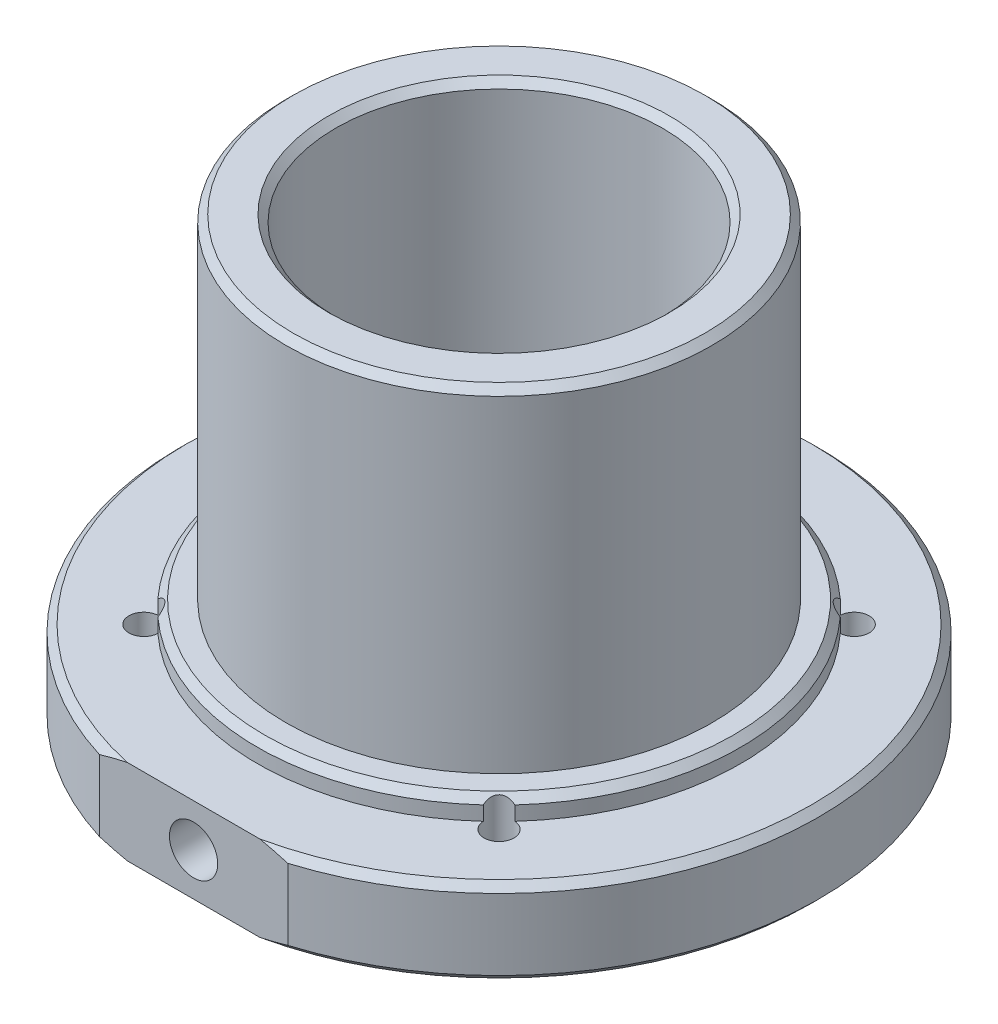
SolidWorks part; units mm, degrees
ref_plane "前视" through (0, 0, 0) normal (0, 0, 1) x (1, 0, 0)
ref_plane "上视" through (0, 0, 0) normal (0, 1, 0) x (1, 0, 0)
ref_plane "右视" through (0, 0, 0) normal (1, 0, 0) x (0, 0, -1)
sketch "草图1" plane through (0, 0, 0) normal (0, 1, 0) x (1, 0, 0)
  circle A0 centre (0, 0) radius 45
  dimension "D1" = 90
extrude "凸台-拉伸1" add sketch "草图1" along normal blind 12
sketch "草图2" plane through (0, 12, 0) normal (0, 1, 0) x (1, 0, 0)
  circle A0 centre (0, 0) radius 30
  dimension "D1" = 60
extrude "凸台-拉伸2" add sketch "草图2" along normal blind 50
cosmetic thread "装饰螺纹线1" parameters "D1"=20, "D2"=58.5
sketch "草图11" plane through (0, 12, 0) normal (0, 1, 0) x (1, 0, 0)
  circle A0 centre (0, 0) radius 34
  dimension "D1" = 68
extrude "凸台-拉伸3" add sketch "草图11" along normal blind 3
sketch "草图3" plane through (0, 0, 0) normal (0, -1, 0) x (1, 0, 0)
  circle A0 centre (0, 0) radius 23
  dimension "D1" = 46
extrude "切除-拉伸1" cut sketch "草图3" against normal through all
chamfer "倒角1" distance 1 angle 45 6 edges at (0, 0, 45) (0, 12, 45) (0, 62, 30) (0, 62, -23) (0, 0, -23) (0, 15, 34)
hole_wizard "M5 螺纹孔1" positions "草图5" profile "草图4" tap size "M5" standard "Gb" end condition through all
sketch "草图5" plane through (0, 0, 0) normal (0, -1, 0) x (-1, 0, 0)
  line L0 (0, 0) -> (0, -37.1797) construction
  line L2 (0, 0) -> (-51.8806, 0) construction
  point P0 (25, -25)
  point P2 (-25, -25)
  point P4 (-25, 25)
  point P6 (25, 25)
  dimension "D1" = 50
  dimension "D2" = 50
sketch "草图4" plane through (-25, 0, 25) normal (1, 0, 0) x (0, 0, -1)
  line L0 (0, 0) -> (0, 62)
  line L1 (0, 62) -> (2.1, 62)
  line L2 (2.1, 62) -> (2.1, 0)
  line L5 (2.1, 0) -> (0, 0)
  line L11 (0, -6.35) -> (0, 107.95) construction
  dimension "通孔螺纹孔钻头直径" = 4.2
  dimension "通孔螺纹孔钻头深度" = 62
cosmetic thread "孔螺蚊线1" parameters "D2"=5
cosmetic thread "孔螺蚊线2" parameters "D2"=5
cosmetic thread "孔螺蚊线3" parameters "D2"=5
cosmetic thread "孔螺蚊线4" parameters "D2"=5
sketch "草图8" plane through (0, 0, 0) normal (0, -1, 0) x (1, 0, 0)
  line L0 (-13.2665, 43) -> (13.2665, 43)
  circle A1 centre (0, 0) radius 45 construction
  arc A2 (13.2665, 43) -> (-13.2665, 43) centre (0, 0) ccw
  dimension "D1" = 43
extrude "切除-拉伸2" cut sketch "草图8" against normal through all
hole_wizard "M8 螺纹孔1" positions "草图10" profile "草图9" tap size "M8" standard "Gb"
sketch "草图10" plane through (0, 0, 43) normal (0, 0, 1) x (1, 0, 0)
  line L0 (-44, 0) -> (44, 0) construction
  point P0 (0, 6)
  dimension "D1" = 6
sketch "草图9" plane through (0, 6, 43) normal (1, 0, 0) x (0, -1, 0)
  line L0 (0, 0) -> (0, 20)
  line L1 (0, 20) -> (3.4, 20)
  line L2 (3.4, 20) -> (3.4, 0)
  line L5 (3.4, 0) -> (0, 0)
  line L11 (0, -6.35) -> (0, 107.95) construction
  dimension "通孔螺纹孔钻头直径" = 6.8
  dimension "通孔螺纹孔钻头深度" = 20
cosmetic thread "孔螺蚊线9" parameters "D2"=8
